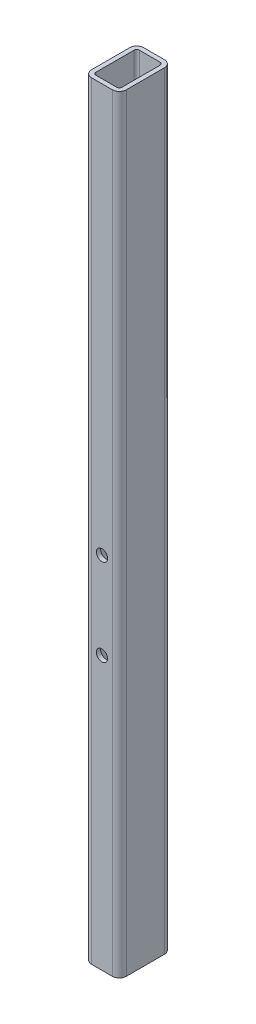
SolidWorks part; units mm, degrees
material "Q235B"
ref_plane "Front Plane" through (0, 0, 0) normal (0, 0, 1) x (1, 0, 0)
ref_plane "Top Plane" through (0, 0, 0) normal (0, 1, 0) x (1, 0, 0)
ref_plane "Right Plane" through (0, 0, 0) normal (1, 0, 0) x (0, 0, -1)
sketch "Sketch1" plane through (0, 0, 0) normal (0, 0, 1) x (1, 0, 0)
  line L0 (0, 0) -> (0, 884)
  dimension "D1" = 884
other "GB/T 6728-2002 rectangular hollow section 60X40X5(1)"
ref_plane "Plane1" through (0, 0, 0) normal (0, 1, 0) x (-1, 0, 0)
sketch "Sketch14" plane through (0, 0, 0) normal (0, 1, 0) x (-1, 0, 0)
  line L0 (-12, -25) -> (12, -25)
  line L1 (-15, -22) -> (-15, 22)
  line L2 (12, 25) -> (-12, 25)
  line L3 (15, 22) -> (15, -22)
  line L4 (-12, -30) -> (12, -30)
  line L5 (-20, -22) -> (-20, 22)
  line L6 (12, 30) -> (-12, 30)
  line L7 (20, 22) -> (20, -22)
  arc A0 (20, 22) -> (12, 30) centre (12, 22) ccw
  arc A1 (12, -30) -> (20, -22) centre (12, -22) ccw
  arc A2 (-20, -22) -> (-12, -30) centre (-12, -22) ccw
  arc A3 (-12, 30) -> (-20, 22) centre (-12, 22) ccw
  arc A4 (-12, 25) -> (-15, 22) centre (-12, 22) ccw
  arc A5 (15, 22) -> (12, 25) centre (12, 22) ccw
  arc A6 (12, -25) -> (15, -22) centre (12, -22) ccw
  arc A7 (-15, -22) -> (-12, -25) centre (-12, -22) ccw
  point P0 (0, 30)
  point P1 (20, 0)
  point P2 (0, -30)
  point P3 (-20, 0)
  point P4 (-20, 30)
  point P5 (20, 30)
  point P6 (20, -30)
  point P7 (-20, -30)
  point P8 (0, 0)
  point P33 (0, 0)
  dimension "D1" = 8
  dimension "Thickness" = 5
  dimension "V_leg" = 60
  dimension "H_leg" = 40
hole_wizard "Ø13.0 (13) Diameter Hole1" positions "Sketch7" profile "Sketch8" hole size "Ø13.0" standard "GB" end condition through all
sketch "Sketch7" plane through (0, 0, 30) normal (0, 0, 1) x (1, 0, 0)
  line L0 (0, 0) -> (0, 314)
  line L1 (0, 314) -> (0, 414)
  line L2 (-12, 884) -> (12, 884) construction
  point P2 (0, 314)
  point P4 (0, 414)
  dimension "D1" = 470
  dimension "D2" = 100
sketch "Sketch8" plane through (0, 414, 30) normal (1, 0, 0) x (0, -1, 0)
  line L0 (0, 0) -> (0, 60)
  line L1 (0, 60) -> (6.5, 60)
  line L2 (6.5, 60) -> (6.5, 0)
  line L5 (6.5, 0) -> (0, 0)
  line L11 (0, -6.35) -> (0, 107.95) construction
  dimension "通孔孔直径" = 13
  dimension "通孔孔深度" = 60
